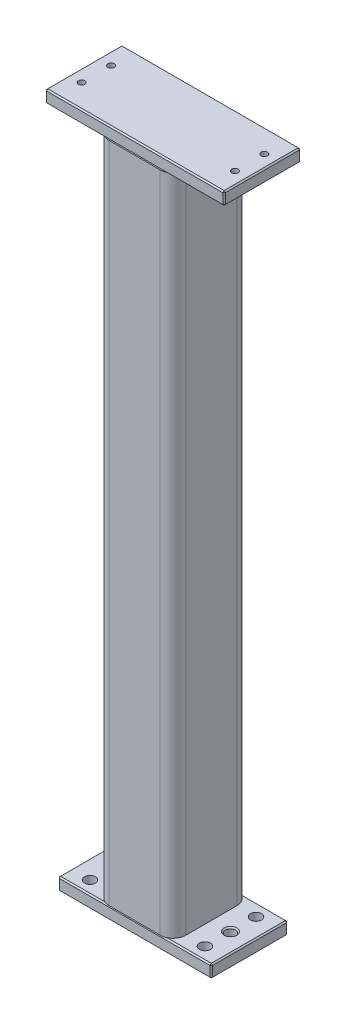
from build123d import *

# Parameters (mm, degrees)
MEMBER_1_DEPTH                   = 519
SKETCH_2_W                       = 140
SKETCH_2_H                       = 60
EXTRUDE_1_DEPTH                  = 10
SKETCH_3_W                       = 120
SKETCH_3_H                       = 60
EXTRUDE_2_DEPTH                  = 10
HOLE_WIZARD_0_AT_2_COUNT         = 2
HOLE_WIZARD_0_AT_2_PITCH         = 120
HOLE_WIZARD_0_AT_3_COUNT         = 2
HOLE_WIZARD_0_AT_3_PITCH         = 122.184287042
HOLE_WIZARD_0_AT_4_COUNT         = 2
HOLE_WIZARD_0_AT_4_PITCH         = 23
CHAMFER_1_SIZE                   = 1
CHAMFER_2_SIZE                   = 1
HOLE_WIZARD_8_6_8_6_1_AT_2_COUNT = 2
HOLE_WIZARD_8_6_8_6_1_AT_2_PITCH = 40
HOLE_WIZARD_8_6_8_6_1_AT_3_COUNT = 2
HOLE_WIZARD_8_6_8_6_1_AT_3_PITCH = 90
HOLE_WIZARD_8_6_8_6_1_AT_4_COUNT = 2
HOLE_WIZARD_8_6_8_6_1_AT_4_PITCH = 98.488578018
SKETCH_9_R                       = 4
CUT_EXTRUDE_1_DEPTH              = 535.45392692
CHAMFER_3_SIZE                   = 1


with BuildPart() as part:
    # Sketch11 → Member 1 (new body)
    with BuildSketch(Plane(origin=(0, 0, 0), x_dir=(1, 0, 0), z_dir=(0, 1, 0))):
        with BuildLine():
            Line((-20, -30), (20, -30))
            ThreePointArc((20, -30), (27.071067812, -27.071067812), (30, -20))
            Line((30, -20), (30, 20))
            ThreePointArc((30, 20), (27.071067812, 27.071067812), (20, 30))
            Line((20, 30), (-20, 30))
            ThreePointArc((-20, 30), (-27.071067812, 27.071067812), (-30, 20))
            Line((-30, 20), (-30, -20))
            ThreePointArc((-30, -20), (-27.071067812, -27.071067812), (-20, -30))
        make_face()
        with BuildLine():
            Line((-20, -25), (20, -25))
            ThreePointArc((20, -25), (23.535533906, -23.535533906), (25, -20))
            Line((25, -20), (25, 20))
            ThreePointArc((25, 20), (23.535533906, 23.535533906), (20, 25))
            Line((20, 25), (-20, 25))
            ThreePointArc((-20, 25), (-23.535533906, 23.535533906), (-25, 20))
            Line((-25, 20), (-25, -20))
            ThreePointArc((-25, -20), (-23.535533906, -23.535533906), (-20, -25))
        make_face(mode=Mode.SUBTRACT)
    extrude(amount=MEMBER_1_DEPTH)


with BuildPart() as body_2:
    # 草图2 → 凸台-拉伸1 (new body)
    with BuildSketch(Plane(origin=(0, 519, 0), x_dir=(1, 0, 0), z_dir=(0, 1, 0))):
        Rectangle(SKETCH_2_W, SKETCH_2_H)
    extrude(amount=EXTRUDE_1_DEPTH)

    # 草图4 → Hole Wizard 0 (revolve, cut)
    with BuildSketch(Plane(origin=(60, 529, -11.5), x_dir=(0, 0, 1), z_dir=(1, 0, 0))):
        Polygon((0, 0), (0, 19.502151548), (2.5, 18), (2.5, 0), align=None)
    hole_wizard_0 = revolve(axis=Axis((60, 535.35, -11.5), (0, -1, 0)), mode=Mode.SUBTRACT)

    # Hole Wizard 0 at 2: Hole Wizard 0 ×2
    with Locations(*[(-i * HOLE_WIZARD_0_AT_2_PITCH, 0, 0) for i in range(1, HOLE_WIZARD_0_AT_2_COUNT)]):
        add(hole_wizard_0, mode=Mode.SUBTRACT)

    # Hole Wizard 0 at 3: Hole Wizard 0 ×2
    with Locations(*[Vector(-0.982123011927037, 0, 0.1882402439526821) * (i * HOLE_WIZARD_0_AT_3_PITCH) for i in range(1, HOLE_WIZARD_0_AT_3_COUNT)]):
        add(hole_wizard_0, mode=Mode.SUBTRACT)

    # Hole Wizard 0 at 4: Hole Wizard 0 ×2
    with Locations(*[(0, 0, i * HOLE_WIZARD_0_AT_4_PITCH) for i in range(1, HOLE_WIZARD_0_AT_4_COUNT)]):
        add(hole_wizard_0, mode=Mode.SUBTRACT)

    # 倒角2
    chamfer_2_edges = [body_2.edges().sort_by_distance(p)[0] for p in [
        (-70, 529, 0),
        (0, 529, 30),
        (70, 529, 0),
        (0, 519, 30),
        (-70, 519, 0),
        (0, 519, -30),
        (70, 519, 0),
        (0, 529, -30),
        (70, 524, 30),
        (-70, 524, 30),
        (-70, 524, -30),
        (70, 524, -30),
    ]]
    chamfer(chamfer_2_edges, length=CHAMFER_2_SIZE)


with BuildPart() as body_3:
    # 草图3 → 凸台-拉伸2 (new body)
    with BuildSketch(Plane.XZ):
        Rectangle(SKETCH_3_W, SKETCH_3_H)
    extrude(amount=EXTRUDE_2_DEPTH)

    # 倒角1
    chamfer_1_edges = [body_3.edges().sort_by_distance(p)[0] for p in [
        (-60, -10, 0),
        (0, -10, -30),
        (60, -10, 0),
        (0, 0, -30),
        (-60, 0, 0),
        (0, 0, 30),
        (60, 0, 0),
        (0, -10, 30),
        (60, -5, -30),
        (-60, -5, -30),
        (-60, -5, 30),
        (60, -5, 30),
    ]]
    chamfer(chamfer_1_edges, length=CHAMFER_1_SIZE)

    # 草图6 → Ø8.6 (8.6) 直径孔1 (revolve, cut)
    with BuildSketch(Plane(origin=(-45, 0, 20), x_dir=(0, 0, 1), z_dir=(1, 0, 0))):
        Polygon((0, 0), (0, 18.092606158), (4.3, 15.61), (4.3, 0), align=None)
    hole_wizard_8_6_8_6_1 = revolve(axis=Axis((-45, 6.35, 20), (0, -1, 0)), mode=Mode.SUBTRACT)

    # Ø8.6 (8.6) 直径孔1 at 2: Ø8.6 (8.6) 直径孔1 ×2
    with Locations(*[(0, 0, -i * HOLE_WIZARD_8_6_8_6_1_AT_2_PITCH) for i in range(1, HOLE_WIZARD_8_6_8_6_1_AT_2_COUNT)]):
        add(hole_wizard_8_6_8_6_1, mode=Mode.SUBTRACT)

    # Ø8.6 (8.6) 直径孔1 at 3: Ø8.6 (8.6) 直径孔1 ×2
    with Locations(*[(i * HOLE_WIZARD_8_6_8_6_1_AT_3_PITCH, 0, 0) for i in range(1, HOLE_WIZARD_8_6_8_6_1_AT_3_COUNT)]):
        add(hole_wizard_8_6_8_6_1, mode=Mode.SUBTRACT)

    # Ø8.6 (8.6) 直径孔1 at 4: Ø8.6 (8.6) 直径孔1 ×2
    with Locations(*[Vector(0.9138115486202572, 0, -0.4061384660534476) * (i * HOLE_WIZARD_8_6_8_6_1_AT_4_PITCH) for i in range(1, HOLE_WIZARD_8_6_8_6_1_AT_4_COUNT)]):
        add(hole_wizard_8_6_8_6_1, mode=Mode.SUBTRACT)

    # 草图9 → 切除-拉伸1 (cut, through all)
    with BuildSketch(Plane(origin=(0, 0, 0), x_dir=(1, 0, 0), z_dir=(0, 1, 0))):
        with Locations(Location((-45, 0, 0), (0, 0, 270))):
            Circle(SKETCH_9_R)
        with Locations(Location((45, 0, 0), (0, 0, 270))):
            Circle(SKETCH_9_R)
    extrude(amount=-CUT_EXTRUDE_1_DEPTH, mode=Mode.SUBTRACT)

    # 倒角3
    chamfer_3_edges = [body_3.edges().sort_by_distance(p)[0] for p in [
        (-45, -10, -4),
        (-45, 0, -4),
        (45, -10, -4),
        (45, 0, -4),
    ]]
    chamfer(chamfer_3_edges, length=CHAMFER_3_SIZE)


solid = Compound([part.part, body_2.part, body_3.part])
